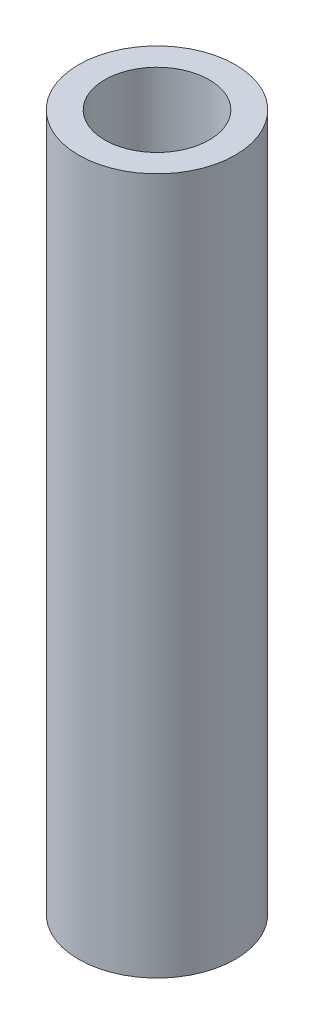
from build123d import *

# Parameters (mm, degrees)
SKETCH1_R           = 2.25
SKETCH1_R_2         = 1.5
BOSS_EXTRUDE1_DEPTH = 20


with BuildPart() as part:
    # Sketch1 → Boss-Extrude1 (new body)
    with BuildSketch(Plane(origin=(0, 0, 0), x_dir=(1, 0, 0), z_dir=(0, 1, 0))):
        with Locations(Location((0, 0, 0), (0, 0, 270))):
            Circle(SKETCH1_R)
        with Locations(Location((0, 0, 0), (0, 0, 270))):
            Circle(SKETCH1_R_2, mode=Mode.SUBTRACT)
    extrude(amount=BOSS_EXTRUDE1_DEPTH)


solid = part.part
